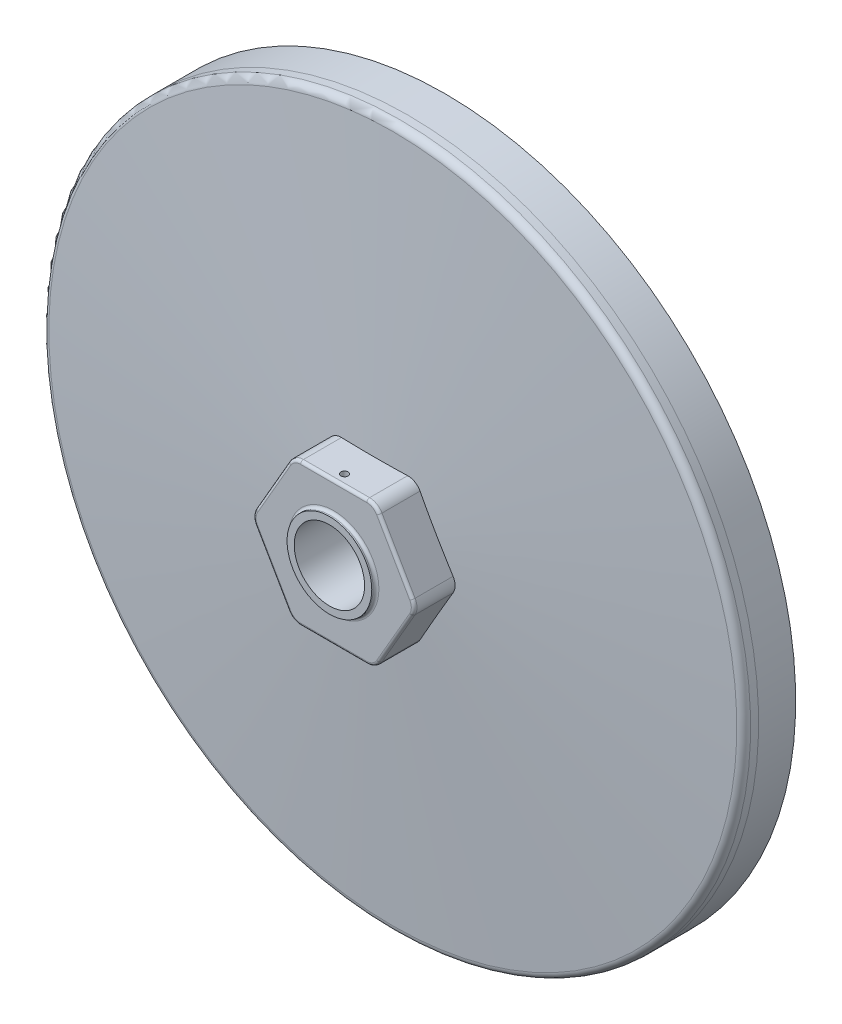
SolidWorks part; units mm, degrees
ref_plane "Front Plane" through (0, 0, 0) normal (0, 0, 1) x (1, 0, 0)
ref_plane "Top Plane" through (0, 0, 0) normal (0, 1, 0) x (1, 0, 0)
ref_plane "Right Plane" through (0, 0, 0) normal (1, 0, 0) x (0, 0, -1)
sketch "Dimension Sketch" plane through (0, 0, 0) normal (0, 0, 1) x (1, 0, 0)
  line L0 (0, 0) -> (24.1005, 0)
  point P3 (6, 0)
  point P5 (11.55, 0)
  point P6 (6.4, 0)
  point P8 (10, 0)
sketch "Sketch1" plane through (0, 0, 0) normal (0, 0, 1) x (1, 0, 0)
  line L0 (-26.8088, 0) -> (37.1748, 0) construction
  line L1 (0, 25.0215) -> (0, -25.0215) construction
  line L3 (2.8875, 5.0013) -> (-2.8875, 5.0013)
  line L4 (-2.8875, 5.0013) -> (-5.775, 0)
  line L5 (-5.775, 0) -> (-2.8875, -5.0013)
  line L6 (-2.8875, -5.0013) -> (2.8875, -5.0013)
  line L7 (2.8875, -5.0013) -> (5.775, 0)
  line L8 (5.775, 0) -> (2.8875, 5.0013)
  circle A0 centre (0, 0) radius 5.0013 construction
  circle A1 centre (0, 0) radius 2.4587
extrude "Boss-Extrude" add sketch "Sketch1" along normal mid plane 6.4
cosmetic thread "Cosmetic Thread1" parameters "D2"=6
sketch "Sketch5" plane through (0, 0, 0) normal (1, 0, 0) x (0, 0, -1)
  line L0 (2.2752, 0) -> (3.964, 24.5025)
  line L1 (2.2752, 0) -> (4.9886, 0)
  line L2 (4.9886, 0) -> (4.9886, 24.5025)
  line L3 (4.9886, 24.5025) -> (3.964, 24.5025)
  line L4 (-3.2, 0) -> (3.2, 0) construction
revolve "Revolve1" add sketch "Sketch5" angle 360 about L1
sketch "Sketch6" plane through (0, 0, 3.2) normal (0, 0, 1) x (1, 0, 0)
  line L6 (5.775, 0) -> (2.8875, 5.0013)
  line L7 (2.8875, 5.0013) -> (-2.8875, 5.0013)
  line L8 (-2.8875, 5.0013) -> (-5.775, 0)
  line L9 (-5.775, 0) -> (-2.8875, -5.0013)
  line L10 (-2.8875, -5.0013) -> (2.8875, -5.0013)
  line L11 (2.8875, -5.0013) -> (5.775, 0)
  line L12 (5.775, 0) -> (2.8875, 5.0013)
  line L13 (2.8875, 5.0013) -> (-2.8875, 5.0013)
  line L14 (-2.8875, 5.0013) -> (-5.775, 0)
  line L15 (-5.775, 0) -> (-2.8875, -5.0013)
  line L16 (-2.8875, -5.0013) -> (2.8875, -5.0013)
  line L17 (2.8875, -5.0013) -> (5.775, 0)
  dimension "D1" = 0
extrude "Cut-Extrude1" cut sketch "Sketch6" against normal blind 3
fillet "Fillet1" radius 0.5 1 edges at (0, -24.5025, -3.964)
fillet "Fillet2" radius 1 6 edges at (-2.8875, -5.0013, -1.2366) (2.8875, -5.0013, -1.2366) (5.775, 0, -1.2366) (-2.8875, 5.0013, -1.2366) (-5.775, 0, -1.2366) (2.8875, 5.0013, -1.2366)
sketch "Sketch7" plane through (0, 0, 0.2) normal (0, 0, 1) x (1, 0, 0)
  circle A0 centre (0, 0) radius 2.4587 construction
  circle A1 centre (0, 0) radius 2.4587
extrude "Extrude-Thin1" add sketch "Sketch7" along normal blind 0.3 thin
fillet "Fillet3" radius 0.2 13 edges at (2.9587, 0, 0.2) (-5.6203, 0, 0.2) (-4.3312, 2.5006, 0.2) (-2.8101, 4.8673, 0.2) (0, 5.0013, 0.2) (2.8101, 4.8673, 0.2) (4.3313, 2.5006, 0.2) (5.6203, 0, 0.2) (4.3312, -2.5006, 0.2) (2.8101, -4.8673, 0.2) (0, -5.0013, 0.2) (-2.8101, -4.8673, 0.2) (-4.3312, -2.5006, 0.2)
sketch "Sketch8" plane through (0, 5.0013, 0) normal (0, 1, 0) x (1, 0, 0)
  circle A0 centre (0, 0.5582) radius 0.25
  dimension "D1" = 0.5
extrude "Cut-Extrude2" cut sketch "Sketch8" against normal blind 4.3 contours A0
sketch "Sketch9" plane through (0, 0, 0) normal (0, 0, 1) x (1, 0, 0)
  circle A0 centre (0, 0) radius 2.4587
extrude "Cut-Extrude3" cut sketch "Sketch9" against normal blind 14.3
scale "Scale1" bodies to scale 112 scale about centroid uniform scaling yes scale factor 2.7
sketch "Sketch10" plane through (0, 0, -6.7145) normal (0, 0, -1) x (-1, 0, 0)
  circle A0 centre (0, 0) radius 66.1578
extrude "Extrude-Thin2" add sketch "Sketch10" along normal blind 7 thin thin type one direction reverse wall 3
equation "\"D2@Cosmetic Thread1\" = \"D@Dimension Sketch\""
equation "\"e@Sketch1\" = \"e@Dimension Sketch\""
equation "\"m@Boss-Extrude\" = \"m@Dimension Sketch\""
